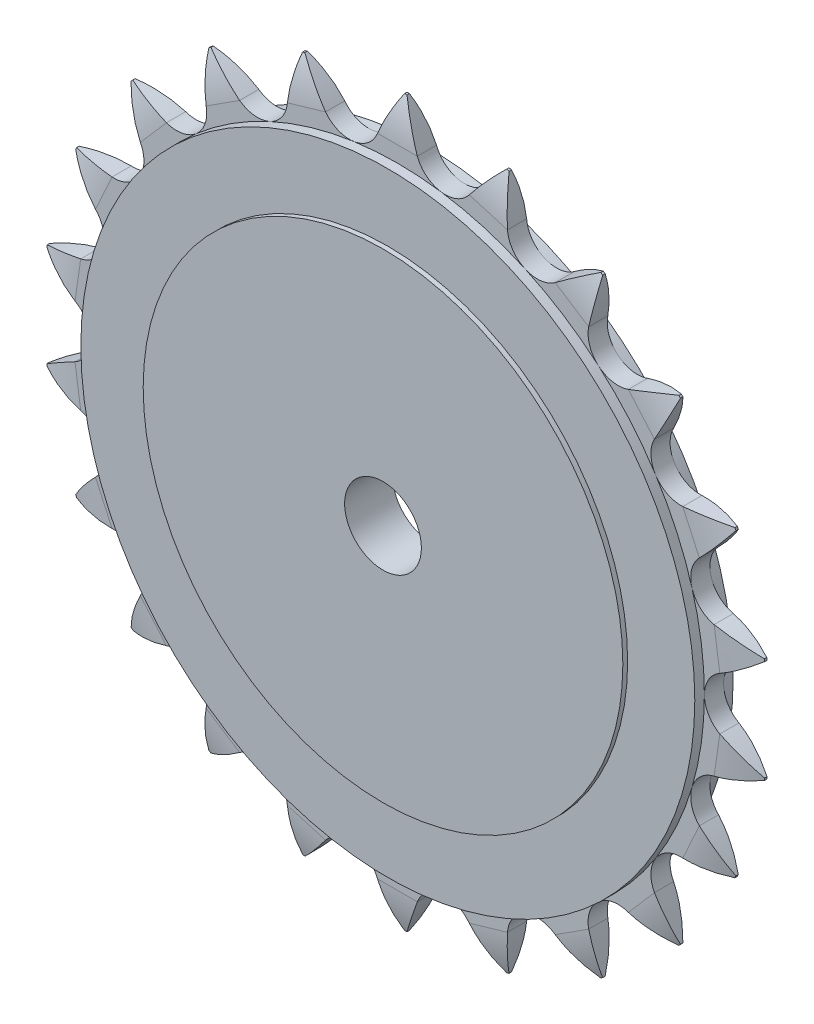
from build123d import *

# Parameters (mm, degrees)
BOSS_EXTRUDE1_DEPTH      = 2
BOSS_EXTRUDE1_DEPTH_BACK = 2
CUT_EXTRUDE1_DEPTH       = 12
CUT_EXTRUDE1_DEPTH_BACK  = 12
CIRPATTERN1_COUNT        = 22
BOSS_EXTRUDE2_DEPTH      = 4
BOSS_EXTRUDE2_DEPTH_BACK = 4
SKETCH5_R                = 64
SKETCH5_R_2              = 50
SKETCH6_R                = 50
BOSS_EXTRUDE3_DEPTH      = 5
SCALE1_SCALE             = 0.5
SCALE2_SCALE             = 0.5
SCALE3_SCALE             = 0.5
SKETCH7_R                = 1
CUT_EXTRUDE2_DEPTH       = 5


with BuildPart() as part:
    # Sketch3 → Boss-Extrude1 (new, two sides: drawn at the far end of the back side and taken through both)
    with BuildSketch(Plane.XY.offset(-BOSS_EXTRUDE1_DEPTH_BACK)):
        with BuildLine():
            Line((-0.25, 75.551527718), (0.25, 75.551527718))
            ThreePointArc((0.25, 75.551527718), (2.354658637, 71.501094858), (4.15, 67.304388564))
            ThreePointArc((4.15, 67.304388564), (6.0916429, 64.652872823), (9.108149649, 63.34857228))
            ThreePointArc((9.108149649, 63.34857228), (0, 64), (-9.108149649, 63.34857228))
            ThreePointArc((-9.108149649, 63.34857228), (-6.0916429, 64.652872823), (-4.15, 67.304388564))
            ThreePointArc((-4.15, 67.304388564), (-2.354658637, 71.501094858), (-0.25, 75.551527718))
        make_face()
    extrude(amount=BOSS_EXTRUDE1_DEPTH + BOSS_EXTRUDE1_DEPTH_BACK)

    # Sketch4 → Cut-Extrude1 (cut, two sides: drawn at the far end of the back side and taken through both)
    with BuildSketch(Plane(origin=(0, 0, 0), x_dir=(0, 0, -1), z_dir=(1, 0, 0)).offset(-CUT_EXTRUDE1_DEPTH_BACK)):
        with BuildLine():
            Line((-0.25, 75.551527718), (0.25, 75.551527718))
            ThreePointArc((0.25, 75.551527718), (1.475155247, 71.502259262), (2, 67.304388564))
            Line((2, 67.304388564), (4.82453427, 67.304388564))
            Line((4.82453427, 67.304388564), (4.82453427, 78.572984978))
            Line((4.82453427, 78.572984978), (-4.812508606, 78.572984978))
            Line((-4.812508606, 78.572984978), (-4.812508606, 67.304388564))
            Line((-4.812508606, 67.304388564), (-2, 67.304388564))
            ThreePointArc((-2, 67.304388564), (-1.475155247, 71.502259262), (-0.25, 75.551527718))
        make_face()
    extrude(amount=CUT_EXTRUDE1_DEPTH + CUT_EXTRUDE1_DEPTH_BACK, mode=Mode.SUBTRACT)


with BuildPart() as cirpattern1_1:
    # CirPattern1: pattern copy
    add(part.part.rotate(Axis((0, 0, 0), (0, 0, 1)), 1 * 360 / CIRPATTERN1_COUNT))


with BuildPart() as cirpattern1_2:
    # CirPattern1: pattern copy
    add(part.part.rotate(Axis((0, 0, 0), (0, 0, 1)), 2 * 360 / CIRPATTERN1_COUNT))


with BuildPart() as cirpattern1_3:
    # CirPattern1: pattern copy
    add(part.part.rotate(Axis((0, 0, 0), (0, 0, 1)), 3 * 360 / CIRPATTERN1_COUNT))


with BuildPart() as cirpattern1_4:
    # CirPattern1: pattern copy
    add(part.part.rotate(Axis((0, 0, 0), (0, 0, 1)), 4 * 360 / CIRPATTERN1_COUNT))


with BuildPart() as cirpattern1_5:
    # CirPattern1: pattern copy
    add(part.part.rotate(Axis((0, 0, 0), (0, 0, 1)), 5 * 360 / CIRPATTERN1_COUNT))


with BuildPart() as cirpattern1_6:
    # CirPattern1: pattern copy
    add(part.part.rotate(Axis((0, 0, 0), (0, 0, 1)), 6 * 360 / CIRPATTERN1_COUNT))


with BuildPart() as cirpattern1_7:
    # CirPattern1: pattern copy
    add(part.part.rotate(Axis((0, 0, 0), (0, 0, 1)), 7 * 360 / CIRPATTERN1_COUNT))


with BuildPart() as cirpattern1_8:
    # CirPattern1: pattern copy
    add(part.part.rotate(Axis((0, 0, 0), (0, 0, 1)), 8 * 360 / CIRPATTERN1_COUNT))


with BuildPart() as cirpattern1_9:
    # CirPattern1: pattern copy
    add(part.part.rotate(Axis((0, 0, 0), (0, 0, 1)), 9 * 360 / CIRPATTERN1_COUNT))


with BuildPart() as cirpattern1_10:
    # CirPattern1: pattern copy
    add(part.part.rotate(Axis((0, 0, 0), (0, 0, 1)), 10 * 360 / CIRPATTERN1_COUNT))


with BuildPart() as cirpattern1_11:
    # CirPattern1: pattern copy
    add(part.part.rotate(Axis((0, 0, 0), (0, 0, 1)), 11 * 360 / CIRPATTERN1_COUNT))


with BuildPart() as cirpattern1_12:
    # CirPattern1: pattern copy
    add(part.part.rotate(Axis((0, 0, 0), (0, 0, 1)), 12 * 360 / CIRPATTERN1_COUNT))


with BuildPart() as cirpattern1_13:
    # CirPattern1: pattern copy
    add(part.part.rotate(Axis((0, 0, 0), (0, 0, 1)), 13 * 360 / CIRPATTERN1_COUNT))


with BuildPart() as cirpattern1_14:
    # CirPattern1: pattern copy
    add(part.part.rotate(Axis((0, 0, 0), (0, 0, 1)), 14 * 360 / CIRPATTERN1_COUNT))


with BuildPart() as cirpattern1_15:
    # CirPattern1: pattern copy
    add(part.part.rotate(Axis((0, 0, 0), (0, 0, 1)), 15 * 360 / CIRPATTERN1_COUNT))


with BuildPart() as cirpattern1_16:
    # CirPattern1: pattern copy
    add(part.part.rotate(Axis((0, 0, 0), (0, 0, 1)), 16 * 360 / CIRPATTERN1_COUNT))


with BuildPart() as cirpattern1_17:
    # CirPattern1: pattern copy
    add(part.part.rotate(Axis((0, 0, 0), (0, 0, 1)), 17 * 360 / CIRPATTERN1_COUNT))


with BuildPart() as cirpattern1_18:
    # CirPattern1: pattern copy
    add(part.part.rotate(Axis((0, 0, 0), (0, 0, 1)), 18 * 360 / CIRPATTERN1_COUNT))


with BuildPart() as cirpattern1_19:
    # CirPattern1: pattern copy
    add(part.part.rotate(Axis((0, 0, 0), (0, 0, 1)), 19 * 360 / CIRPATTERN1_COUNT))


with BuildPart() as cirpattern1_20:
    # CirPattern1: pattern copy
    add(part.part.rotate(Axis((0, 0, 0), (0, 0, 1)), 20 * 360 / CIRPATTERN1_COUNT))


with BuildPart() as cirpattern1_21:
    # CirPattern1: pattern copy
    add(part.part.rotate(Axis((0, 0, 0), (0, 0, 1)), 21 * 360 / CIRPATTERN1_COUNT))


with BuildPart() as part_1:
    add(part.part)

    add(cirpattern1_1.part)  # Boss-Extrude2 merges CirPattern1_1

    add(cirpattern1_2.part)  # Boss-Extrude2 merges CirPattern1_2

    add(cirpattern1_3.part)  # Boss-Extrude2 merges CirPattern1_3

    add(cirpattern1_4.part)  # Boss-Extrude2 merges CirPattern1_4

    add(cirpattern1_5.part)  # Boss-Extrude2 merges CirPattern1_5

    add(cirpattern1_6.part)  # Boss-Extrude2 merges CirPattern1_6

    add(cirpattern1_7.part)  # Boss-Extrude2 merges CirPattern1_7

    add(cirpattern1_8.part)  # Boss-Extrude2 merges CirPattern1_8

    add(cirpattern1_9.part)  # Boss-Extrude2 merges CirPattern1_9

    add(cirpattern1_10.part)  # Boss-Extrude2 merges CirPattern1_10

    add(cirpattern1_11.part)  # Boss-Extrude2 merges CirPattern1_11

    add(cirpattern1_12.part)  # Boss-Extrude2 merges CirPattern1_12

    add(cirpattern1_13.part)  # Boss-Extrude2 merges CirPattern1_13

    add(cirpattern1_14.part)  # Boss-Extrude2 merges CirPattern1_14

    add(cirpattern1_15.part)  # Boss-Extrude2 merges CirPattern1_15

    add(cirpattern1_16.part)  # Boss-Extrude2 merges CirPattern1_16

    add(cirpattern1_17.part)  # Boss-Extrude2 merges CirPattern1_17

    add(cirpattern1_18.part)  # Boss-Extrude2 merges CirPattern1_18

    add(cirpattern1_19.part)  # Boss-Extrude2 merges CirPattern1_19

    add(cirpattern1_20.part)  # Boss-Extrude2 merges CirPattern1_20

    add(cirpattern1_21.part)  # Boss-Extrude2 merges CirPattern1_21
    # Sketch5 → Boss-Extrude2 (add, two sides: drawn at the far end of the back side and taken through both)
    with BuildSketch(Plane.XY.offset(-BOSS_EXTRUDE2_DEPTH_BACK)):
        Circle(SKETCH5_R)
        Circle(SKETCH5_R_2, mode=Mode.SUBTRACT)
    extrude(amount=BOSS_EXTRUDE2_DEPTH + BOSS_EXTRUDE2_DEPTH_BACK)

    # Sketch6 → Boss-Extrude3 (add, symmetric)
    with BuildSketch(Plane.XY):
        Circle(SKETCH6_R)
    extrude(amount=BOSS_EXTRUDE3_DEPTH, both=True)


with BuildPart() as part_2:
    # Scale1: scaled about (0, 0, 0)
    add(part_1.part.scale(SCALE1_SCALE))


with BuildPart() as part_3:
    # Scale2: scaled about (0, 0, 0)
    add(part_2.part.scale(SCALE2_SCALE))


with BuildPart() as part_4:
    # Scale3: scaled about (0, 0, 0)
    add(part_3.part.scale(SCALE3_SCALE))

    # Sketch7 → Cut-Extrude2 (cut, symmetric)
    with BuildSketch(Plane.XY):
        Circle(SKETCH7_R)
    extrude(amount=CUT_EXTRUDE2_DEPTH, both=True, mode=Mode.SUBTRACT)


solid = part_4.part
